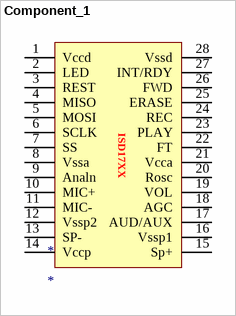
[diagram p0: symbol Component_1]
# Altium schematic symbol library MISC86338-4.SchLib: 1 symbol
Pins are listed as number, name and electrical type; pins without a type are passive.


## Component_1
designator *
footprint ISD1730
pins: 1 Vccd, 2 LED, 3 REST, 4 MISO, 5 MOSI, 6 SCLK, 7 SS, 8 Vssa, 9 Analn, 10 MIC+, 11 MIC-, 12 Vssp2, 13 SP-, 14 Vccp, 15 Sp+, 16 Vssp1, 17 AUD/AUX, 18 AGC, 19 VOL, 20 Rosc, 21 Vcca, 22 FT, 23 PLAY, 24 REC, 25 ERASE, 26 FWD, 27 INT/RDY, 28 Vssd